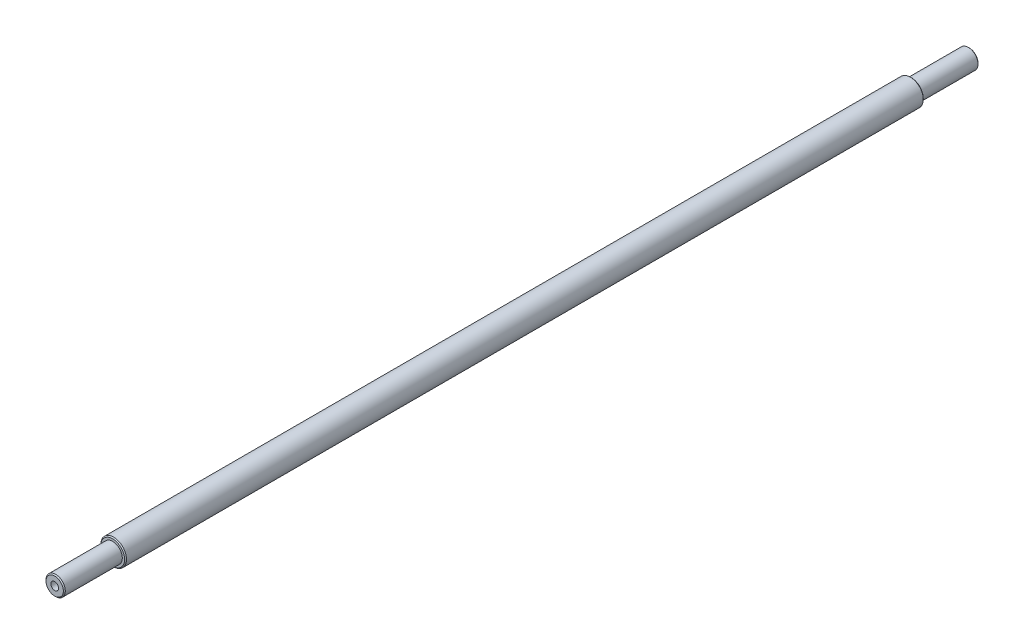
from build123d import *

# Parameters (mm, degrees)
SKETCH1_R              = 15
BOSS_EXTRUDE1_DEPTH    = 710
M14_TAPPED_HOLE2_D     = 12
M14_TAPPED_HOLE2_DEPTH = 34
M14_TAPPED_HOLE2_TIP   = 3.605163714
M14_TAPPED_HOLE1_D     = 12
M14_TAPPED_HOLE1_DEPTH = 34
M14_TAPPED_HOLE1_TIP   = 3.605163714
SKETCH7_R              = 20
BOSS_EXTRUDE3_DEPTH    = 620
CHAMFER1_SIZE          = 1.5


with BuildPart() as part:
    # Sketch1 → Boss-Extrude1 (new, symmetric)
    with BuildSketch(Plane.XY):
        Circle(SKETCH1_R)
    extrude(amount=BOSS_EXTRUDE1_DEPTH, both=True)

    # M14 Tapped Hole2
    with Locations(Plane.XY.offset(710)):
        with Locations((0, 0)):
            Hole(M14_TAPPED_HOLE2_D / 2, depth=M14_TAPPED_HOLE2_DEPTH)
            with Locations((0, 0, -(M14_TAPPED_HOLE2_DEPTH + M14_TAPPED_HOLE2_TIP / 2))):  # 118° drill point
                Cone(0, M14_TAPPED_HOLE2_D / 2, M14_TAPPED_HOLE2_TIP, mode=Mode.SUBTRACT)

    # M14 Tapped Hole1
    with Locations(Plane(origin=(0, 0, -710), x_dir=(-1, 0, 0), z_dir=(0, 0, -1))):
        with Locations((0, 0)):
            Hole(M14_TAPPED_HOLE1_D / 2, depth=M14_TAPPED_HOLE1_DEPTH)
            with Locations((0, 0, -(M14_TAPPED_HOLE1_DEPTH + M14_TAPPED_HOLE1_TIP / 2))):  # 118° drill point
                Cone(0, M14_TAPPED_HOLE1_D / 2, M14_TAPPED_HOLE1_TIP, mode=Mode.SUBTRACT)

    # Sketch7 → Boss-Extrude3 (add, symmetric)
    with BuildSketch(Plane.XY):
        Circle(SKETCH7_R)
    extrude(amount=BOSS_EXTRUDE3_DEPTH, both=True)

    # Chamfer1
    chamfer1_edges = [part.edges().sort_by_distance(p)[0] for p in [
        (-20, 0, -620),
        (-20, 0, 620),
        (-15, 0, -710),
        (-15, 0, 710),
    ]]
    chamfer(chamfer1_edges, length=CHAMFER1_SIZE)


solid = part.part
